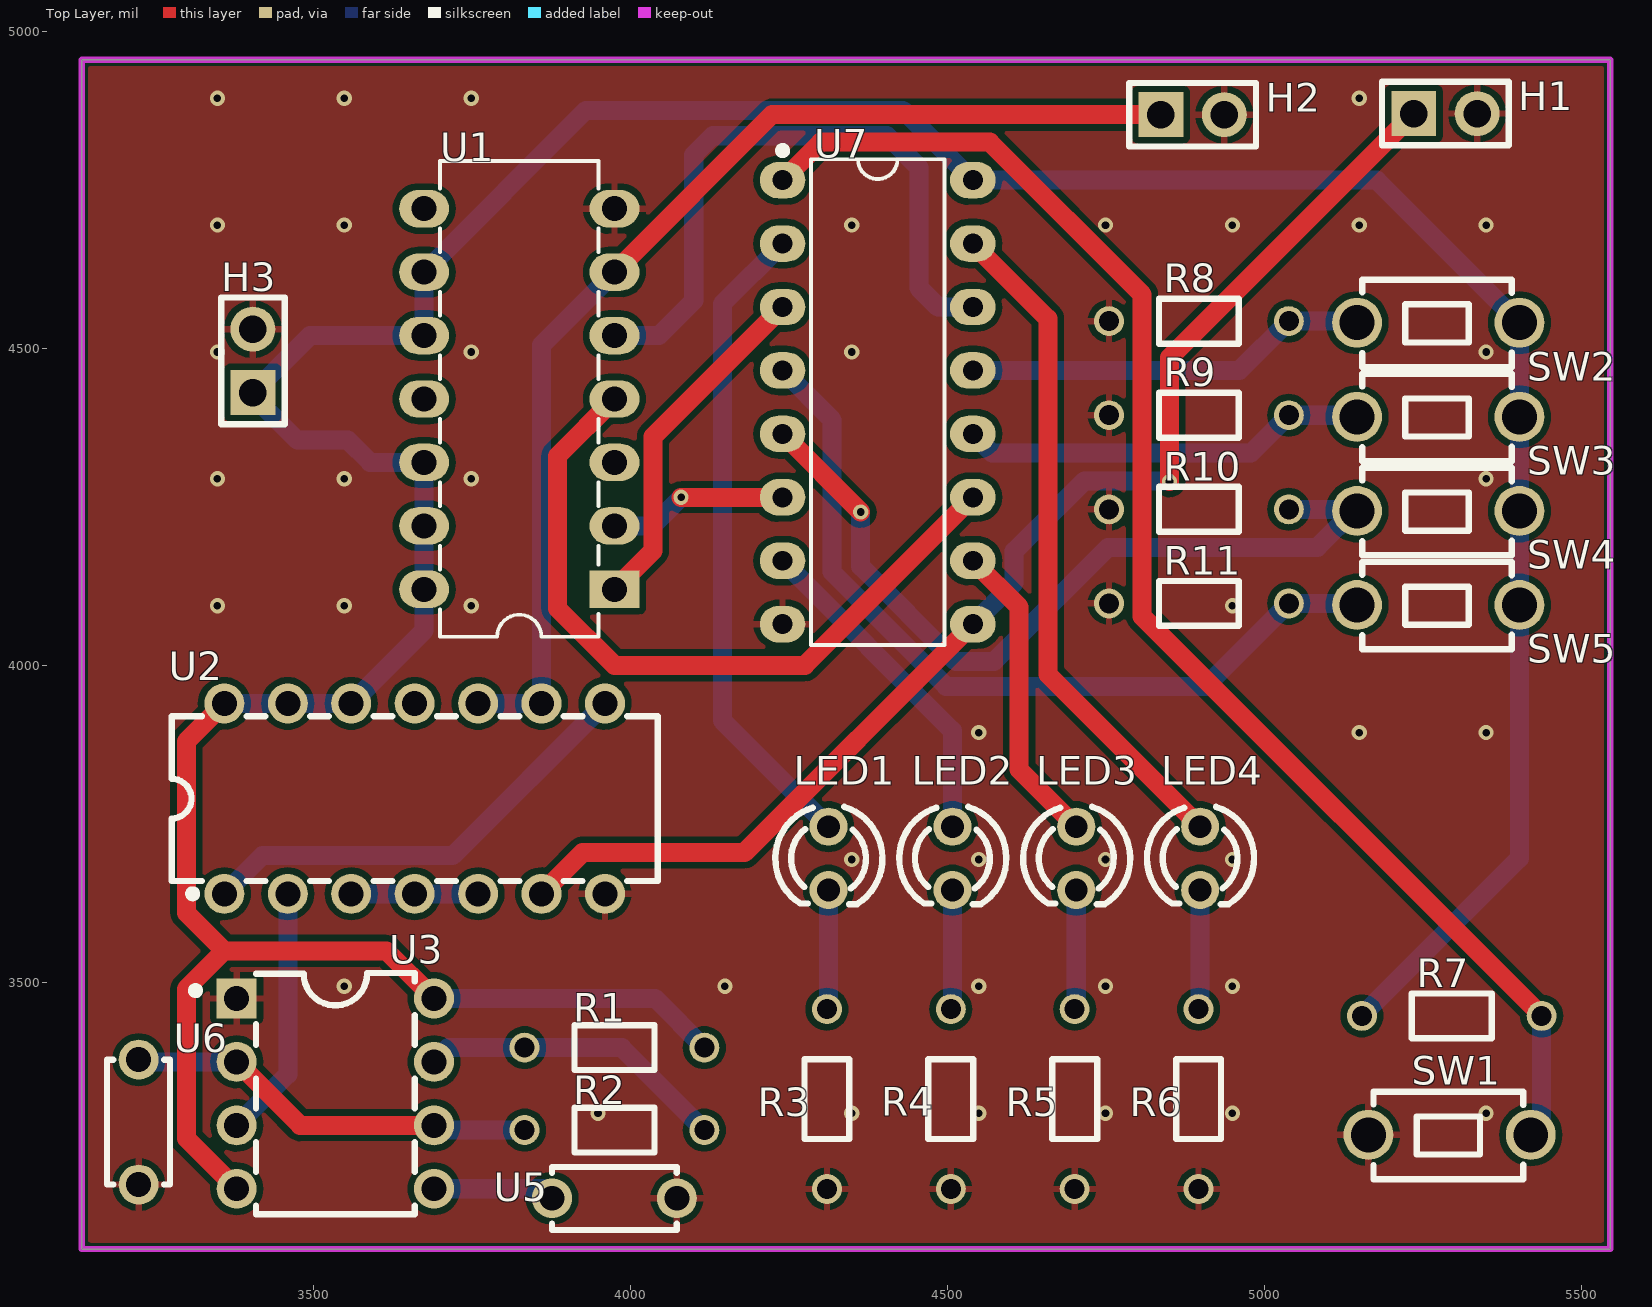
[diagram p0: Top Layer view]
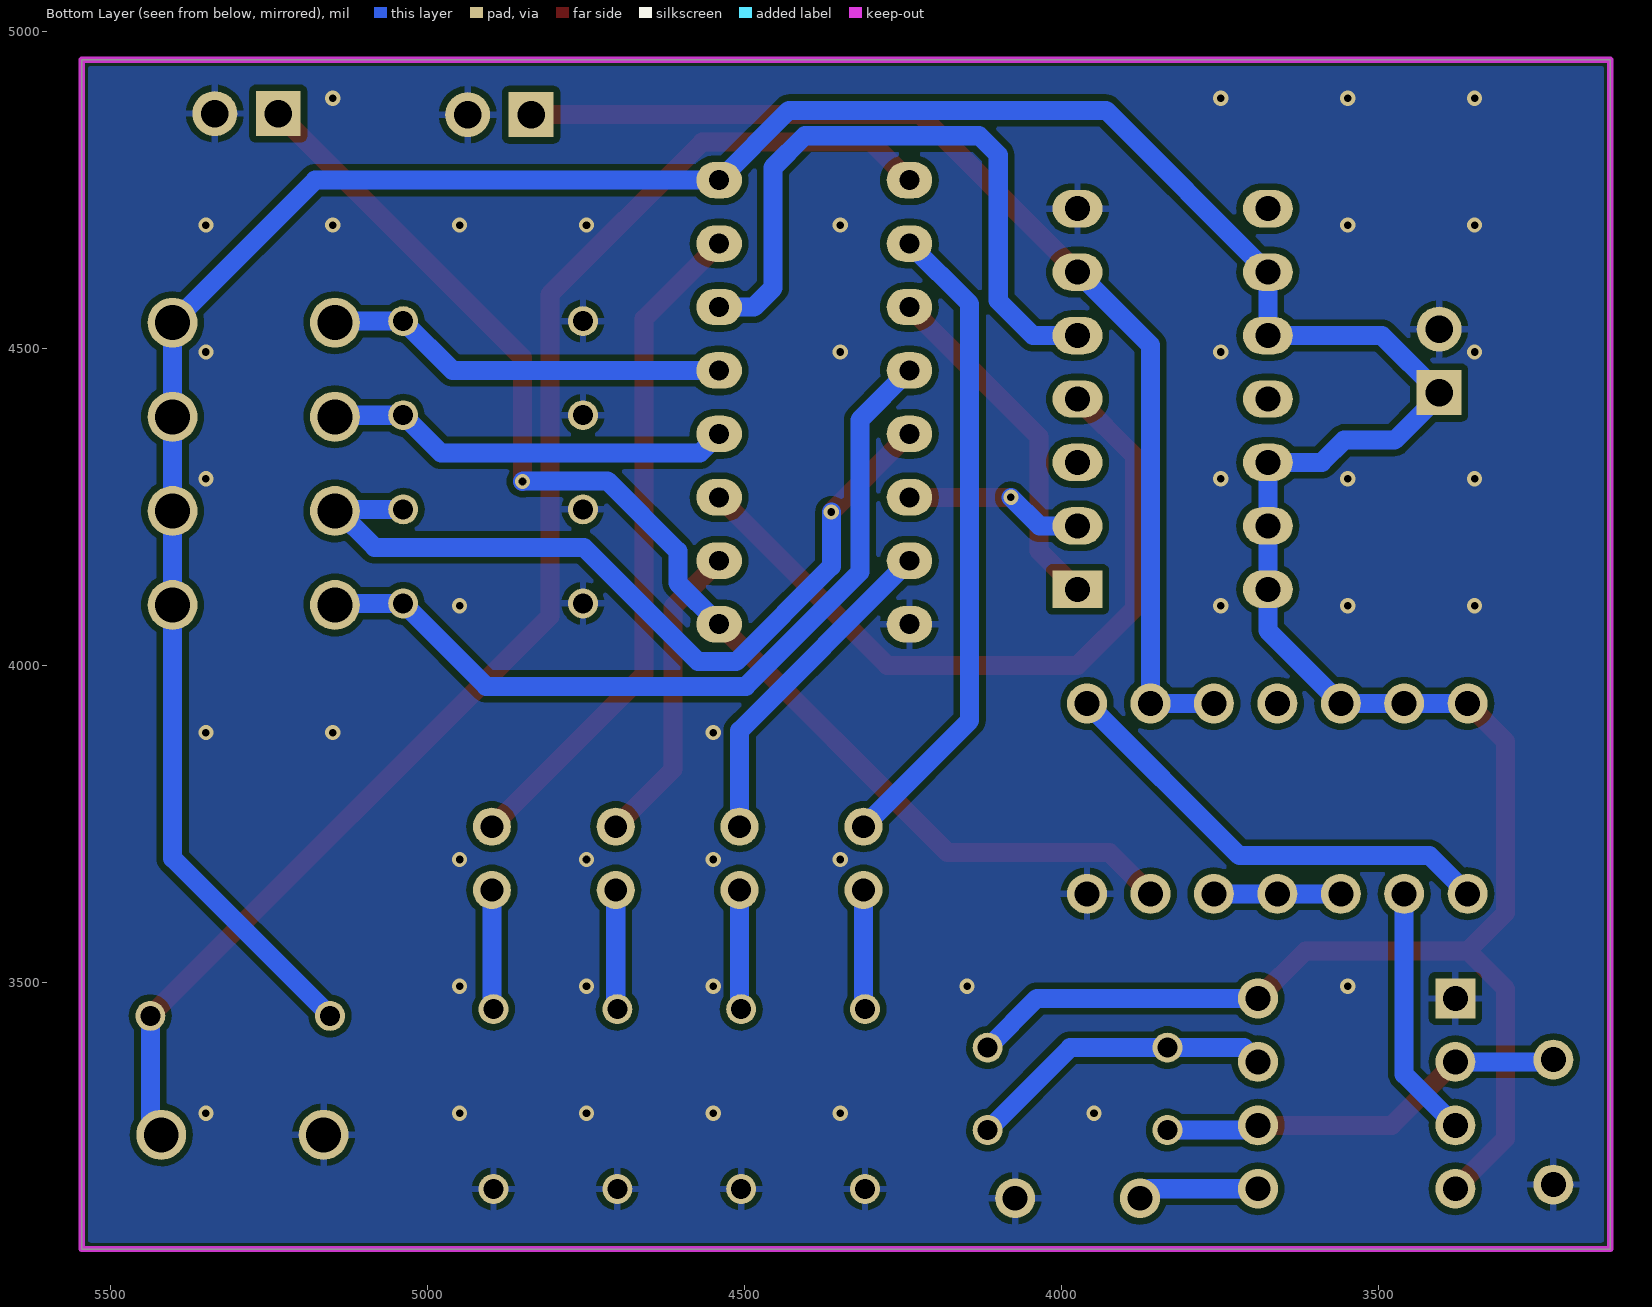
[diagram p1: Bottom Layer view, seen from below]
# Altium PCB MISC49856.pcbdoc
Units mil, origin at the board's own origin, x right, y up, seen from the top; angles counter-clockwise.
Board outline 2410 x 1875 mil, 2 copper layers (Top Layer, Bottom Layer), stack 62.206 mil thick; 29 components, 27 nets, 102 pads, 44 vias.

## Layer stack, top to bottom
Top Solder Mask Layer: solder mask 0.394, Dk 3.3
Top Layer: signal copper 1.379
Dielectric1: surface 59.449, FR4, Dk 4.5
Bottom Layer: signal copper 1.378
Bottom Solder Mask Layer: solder mask 0.394, Dk 3.3

## Board outline
3135,4955 3135,3080 5545,3080 5545,4955

## Design rules (kind name [scope] priority, off if disabled: settings)
BoardOutlineClearance copperThickness2oz_1 [All] p2 off: genericclearance=7.99 ignorepadtopadclearanceinfootprint=FALSE except(0: Arc-SplitContinuation Track-SplitContinuation SMDPad-SplitContinuation THPad-SplitContinuation Via-SplitContinuation Fill-SplitContinuation Region-SplitContinuation Poly-SplitContinuation Text-SplitContinuation Hole-SplitContinuation; 5.98: Arc-CutoutEdge SMDPad-CutoutEdge THPad-CutoutEdge Via-CutoutEdge Fill-CutoutEdge Region-CutoutEdge Text-CutoutEdge; 6.93: Hole-OutlineEdge Hole-CutoutEdge; 10: Poly-OutlineEdge Poly-CutoutEdge; 11.81: Arc-OutlineEdge Track-OutlineEdge SMDPad-OutlineEdge THPad-OutlineEdge Via-OutlineEdge Fill-OutlineEdge Region-OutlineEdge Text-OutlineEdge Track-CutoutEdge)
BoardOutlineClearance copperThickness1oz_1 [All] p4: genericclearance=4.02 ignorepadtopadclearanceinfootprint=FALSE except(0: Arc-SplitContinuation Track-SplitContinuation SMDPad-SplitContinuation THPad-SplitContinuation Via-SplitContinuation Fill-SplitContinuation Region-SplitContinuation Poly-SplitContinuation Text-SplitContinuation Hole-SplitContinuation; 6: SMDPad-CutoutEdge THPad-CutoutEdge Via-CutoutEdge Fill-CutoutEdge Region-CutoutEdge Text-CutoutEdge; 6.93: Hole-OutlineEdge Hole-CutoutEdge; 10: Poly-OutlineEdge Poly-CutoutEdge; 11.8: Arc-OutlineEdge Track-OutlineEdge SMDPad-OutlineEdge THPad-OutlineEdge Via-OutlineEdge Fill-OutlineEdge Region-OutlineEdge Text-OutlineEdge; 11.81: Arc-CutoutEdge Track-CutoutEdge)
Clearance copperThickness2oz [All] p1 off: gap=7.99 ignorepadtopadclearanceinfootprint=FALSE except(5.98: SMDPad-Track SMDPad-SMDPad THPad-Track SMDPad-THPad THPad-THPad Track-Via SMDPad-Via THPad-Via Via-Via Fill-Track Region-Track Fill-SMDPad Region-SMDPad Fill-THPad Region-THPad Fill-Via Region-Via Fill-Fill Fill-Region Region-Region Arc-Track Arc-SMDPad Arc-THPad Arc-Via Fill-Arc Region-Arc Arc-Arc Text-Track SMDPad-Text Text-THPad Text-Via Fill-Text Region-Text Arc-Text Text-Text; 6.93: Hole-Track Hole-SMDPad Hole-THPad Hole-Via Fill-Hole Region-Hole Hole-Arc Hole-Text; 10: Poly-Track Poly-SMDPad Poly-THPad Poly-Via Poly-Fill Poly-Region Poly-Poly Poly-Arc Poly-Text Poly-Hole)
Clearance copperThickness1oz [All] p3: gap=4.02 ignorepadtopadclearanceinfootprint=FALSE except(5.98: SMDPad-Track SMDPad-SMDPad THPad-Track SMDPad-THPad THPad-THPad Track-Via SMDPad-Via THPad-Via Via-Via Fill-Track Region-Track Fill-SMDPad Region-SMDPad Fill-THPad Region-THPad Fill-Via Region-Via Fill-Fill Fill-Region Region-Region; 6: Arc-Track Arc-SMDPad Arc-THPad Arc-Via Fill-Arc Region-Arc Arc-Arc Text-Track SMDPad-Text Text-THPad Text-Via Fill-Text Region-Text Arc-Text Text-Text; 6.93: Hole-Track Hole-SMDPad Hole-THPad Hole-Via Fill-Hole Region-Hole Hole-Arc Hole-Text; 10: Poly-Track Poly-SMDPad Poly-THPad Poly-Via Poly-Fill Poly-Region Poly-Poly Poly-Arc Poly-Text Poly-Hole)
Creepage creepage [All] p1: checkdistance=0 ignoreinternallayers=TRUE applytopolygonpour=TRUE
DiffPairsRouting differentialPair [All] p1: maxlimit=6 minlimit=6 mostfreqgap=6 toplayer_minwidth=5 toplayer_prefwidth=10 toplayer_maxwidth=100 toplayer_mingap=6 toplayer_prefgap=6 toplayer_maxgap=6 bottomlayer_minwidth=5 bottomlayer_prefwidth=10 bottomlayer_maxwidth=100 bottomlayer_mingap=6 bottomlayer_prefgap=6 bottomlayer_maxgap=6 maxuncoupledlength=10
HoleToHoleClearance otherClearance [All] p1: gap=11.81 allowstackedmicrovias=TRUE
Length netLength [All] p1: minlimit=0 maxlimit=0
MatchedLengths netLengthTolerance [All] p1: tolerance=1000
PasteMaskExpansion pasteMaskExpansion [All] p1: expansion=0
PlaneConnect innerPlane [All] p1: planeconnectstyle=Relief reliefexpansion=20 reliefentries=4 reliefconductorwidth=10 reliefairgap=10
PolygonConnect copperRegion [(InNet('GND'))] p1: connectstyle=Relief reliefconductorwidth=10 reliefentries=4 polygonreliefangle="90 Angle" airgapwidth=10 via.connectstyle=Relief via.reliefconductorwidth=10 via.reliefentries=4 via.polygonreliefangle="90 Angle" via.airgapwidth=10
RoutingVias viaSize [All] p1: holewidth=12.01 width=24.02 viastyle="Through Hole" minholewidth=11.81 minwidth=19.68 maxholewidth=248.03 maxwidth=393.7
SolderMaskExpansion solderMaskExpansion [IsVia] p1: expansion=-1000 istentingtop=TRUE
SolderMaskExpansion solderMaskExpansion [All] p2: expansion=2 istentingtop=FALSE
Width copperThickness2oz_2 [All] p1 off: maxlimit=100 minlimit=8 preferedwidth=10
Width copperThickness1oz_2 [All] p2: maxlimit=10 minlimit=10 preferedwidth=10 toplayer_minwidth=30 toplayer_maxwidth=100 toplayer_prefwidth=30 bottomlayer_minwidth=30 bottomlayer_maxwidth=100 bottomlayer_prefwidth=30

## Components (designator, comment, footprint, x,y, rotation, side; value= is the part's Value field where it differs from the comment)
H1 "" HDR-TH_2P-P2.54-V-M-1 5285,4870 r0 top
H2 "" HDR-TH_2P-P2.54-V-M-1 4886.33,4868.15 r0 top
H3 "" HDR-TH_2P-P2.54-V-M-1 3405,4480 r90 top
LED1 "" LED_TH-3mm 4312.42,3695.79 r270 top
LED2 "" LED_TH-3mm 4507.71,3695.79 r270 top
LED3 "" LED_TH-3mm 4702.99,3695.79 r270 top
LED4 "" LED_TH-3mm 4898.28,3695.79 r270 top
R1 "4.3kΩ" Res_1/8W 3975,3395 r0 top
R2 "5.1kΩ" Res_1/8W 3975,3265 r0 top
R3 "220Ω" Res_1/8W 4312.42,3316.4 r90 top
R4 "220Ω" Res_1/8W 4507.71,3316.4 r90 top
R5 "220Ω" Res_1/8W 4702.99,3316.4 r90 top
R6 "220Ω" Res_1/8W 4898.28,3316.4 r90 top
R7 "10kΩ" Res_1/8W 5295,3445 r0 top
R8 "10kΩ" Res_1/8W 4896.35,4540.24 r0 top
R9 "10kΩ" Res_1/8W 4896.35,4391.91 r0 top
R10 "10kΩ" Res_1/8W 4896.35,4243.59 r0 top
R11 "10kΩ" Res_1/8W 4896.35,4095.26 r0 top
SW1 "" Key_TH_3.5x6x4.3 5285,3260 r0 top
SW2 "" Key_TH_3.5x6x4.3 5267.12,4540.24 r0 top
SW3 "" Key_TH_3.5x6x4.3 5267.12,4391.91 r0 top
SW4 "" Key_TH_3.5x6x4.3 5267.12,4243.59 r0 top
SW5 "" Key_TH_3.5x6x4.3 5267.12,4095.26 r0 top
U1 "SN74LS20N(XBLW)" DIP-14_L19.0-W6.4-P2.54-LS7.6-BL 3825,4420 r90 top
U2 "SN74LS00NE4" PDIP-14_L19.3-W6.4-P2.54-LS7.9-BL 3660,3790 r0 top
U3 "LM555CM" PDIP-8_L9.6-W6.4-P2.54-LS7.9-BL-1 3535,3325 r270 top
U5 "10nF" CAP-TH_L5.0-W2.5-P5.00-D1.0 3975,3160 r0 top
U6 "100nF" CAP-TH_L5.0-W2.5-P5.00-D1.0 3225,3280 r270 top
U7 "SN74LS175N" DIP-16_L19.3-W6.4-P2.54-LS7.6-BL 4390,4415 r270 top

## Footprints (in the part's own frame and the unit in brackets; to place one, negate y for a bottom-side part, rotate by r counter-clockwise, add the part's x,y. Pads: shape width x height; smd on the part's side, far side on the other; paste and mask are expansions set on the pad)
CAP-TH_L5.0-W2.5-P5.00-D1.0 [mm]
  round 1.6 hole 1: 1(-2.5,0) 2(2.5,0)
  silkscreen extent -2.5,-1.27 2.5,1.25
DIP-14_L19.0-W6.4-P2.54-LS7.6-BL [mm]
  rect 1.5x2 hole 1: 1(-7.62,-3.81)
  oval 1.5x2 hole 1: 2(-5.08,-3.81) 3(-2.54,-3.81) 4(0,-3.81) 5(2.54,-3.81) 6(5.08,-3.81) 7(7.62,-3.81) 8(7.62,3.81) 9(5.08,3.81) 10(2.54,3.81) 11(0,3.81) 12(-2.54,3.81) 13(-5.08,3.81) 14(-7.62,3.81)
  silkscreen extent -9.53,-3.18 9.53,3.18
DIP-16_L19.3-W6.4-P2.54-LS7.6-BL [mm]
  oval 1.46x1.825 hole 0.8: 1(-8.89,-3.81) 2(-6.35,-3.81) 3(-3.81,-3.81) 4(-1.27,-3.81) 5(1.27,-3.81) 6(3.81,-3.81) 7(6.35,-3.81) 8(8.89,-3.81) 9(8.89,3.81) 10(6.35,3.81) 11(3.81,3.81) 12(1.27,3.81) 13(-1.27,3.81) 14(-3.81,3.81) 15(-6.35,3.81) 16(-8.89,3.81)
  silkscreen extent -10.22,-3.96 9.73,2.67
HDR-TH_2P-P2.54-V-M-1 [mm]
  rect 1.8x1.8 hole 1.1: 1(-1.27,0)
  round 1.8 hole 1.1: 2(1.27,0)
  silkscreen extent -2.54,-1.27 2.54,1.27
Key_TH_3.5x6x4.3 [mil]
  round 78.7 hole 55.1 paste+0 mask+2: A(-121.44,0) B(134.46,0)
  silkscreen extent -114,-70 123,68
LED_TH-3mm [mil]
  round 60 hole 36 paste+0 mask+2: 1(-50,0) 2(50,0)
  silkscreen extent -81,-84 72,85
PDIP-8_L9.6-W6.4-P2.54-LS7.9-BL-1 [mil]
  rect 63x63 hole 39.37: 1(-150,-155.51)
  round 63 hole 39.37: 2(-50,-155.51) 3(50,-155.51) 4(150,-155.51) 5(150,155.52) 6(50,155.52) 7(-50,155.52) 8(-150,155.52)
  silkscreen extent -190,-226 190,125
PDIP-14_L19.3-W6.4-P2.54-LS7.9-BL [mm]
  round 1.6 hole 1: 1(-7.62,-3.81) 2(-5.08,-3.81) 3(-2.54,-3.81) 4(0,-3.81) 5(2.54,-3.81) 6(5.08,-3.81) 7(7.62,-3.81) 8(7.62,3.81) 9(5.08,3.81) 10(2.54,3.81) 11(0,3.81) 12(-2.54,3.81) 13(-5.08,3.81) 14(-7.62,3.81)
  silkscreen extent -9.73,-3.96 9.73,3.3
Res_1/8W [mil]
  round 47.2 hole 31.5 paste+0 mask+2: 1(-141.7,2.48) 2(141.7,2.48)
  silkscreen extent -63,-33 63,38

## Via types
v1: diameter 24.02, hole 12, Top Layer to Bottom Layer, 44 vias

## Nets (pads, with @x,y where several pads share a name; then routed paths per layer and width w, separated by ;. In a path a pad name is that pad's centre, name@x,y a point inside that pad or via, vN(x,y) a via of type N, cw(c..) or ccw(c..) an arc to the next point about the centre after c; other vN are vias at no path point)
$1N1: U2.2 U3.3 | length 398.3
  Bottom Layer w30: U3.3 3460,3355.52 U2.2
$1N2: R1.1 R2.2 U3.7 | length 489.3
  Bottom Layer w30: U3.7 3712.99,3397.48 R1.1 3986.7,3397.48 R2.2
$1N4: R2.1 U3.2 U3.6 U6.1 | length 654.3
  Top Layer w30: U3.2 3479.49,3275 U3.6
  Bottom Layer w30: U6.1 3228.42,3375 U3.2 ; U3.6 3698.03,3267.48 R2.1
$1N5: U3.5 U5.1 | length 192.3
  Bottom Layer w30: U3.5 3861.58,3175 U5.1
$1N7: LED1.2 R3.2 | length 188.7
  Bottom Layer w30: R3.2 4312.42,3460.58 LED1.2
$1N8: LED2.2 R4.2 | length 188.7
  Bottom Layer w30: R4.2 4507.71,3460.58 LED2.2
$1N9: LED3.2 R5.2 | length 188.7
  Bottom Layer w30: R5.2 4702.99,3460.58 LED3.2
$1N10: LED4.2 R6.2 | length 188.7
  Bottom Layer w30: R6.2 4898.28,3460.58 LED4.2
$1N11: LED4.1 U7.15 | length 1067.6
  Top Layer w30: U7.15 4658.28,4546.72 4658.28,3985.79 LED4.1
$1N12: LED3.1 U7.10 | length 486.7
  Top Layer w30: U7.10 4612.99,4092.01 4612.99,3835.79 LED3.1
$1N13: LED2.1 U7.7 | length 530.1
  Bottom Layer w30: U7.7 4507.71,3897.29 LED2.1
$1N14: LED1.1 U7.2 | length 1027.9
  Bottom Layer w30: U7.2 4145,4570 4145,3913.21 LED1.1
$1N15: U1.1 U7.3 | length 554.8
  Top Layer w30: U1.1 4035.75,4180.75 4035.75,4360.75 U7.3
$1N16: U1.2 U7.6 | length 283.6
  Top Layer w30: v1(4080,4265) U7.6
  Bottom Layer w30: U1.2 4035,4220 v1(4080,4265)
$1N17: U1.4 U7.11 | length 1169.3
  Top Layer w30: U1.4 3885,4330 3885,4090 3975,4000 4275,4000 U7.11
$1N18: U1.5 U7.14 | length 1053.3
  Bottom Layer w30: U1.5 4045,4520 4100,4575 4100,4805 4130,4835 4210.77,4835 4405,4835 4455,4785 4455,4595 4485,4565 U7.14
$1N19: R7.2 SW1.B U7.1 | length 2284.1
  Top Layer w30: U7.1 4300,4825 4566.7,4825 4806.7,4585 4806.7,4077.47 R7.2
  Bottom Layer w30: SW1.B 5436.7,3277.24 R7.2
$1N20: H1.1 U2.6 U7.9 | length 2028.5
  Top Layer w30: U2.6 3925.01,3705 4180,3705 U7.9 ; v1(4850,4290) 4850,4485 H1.1
  Bottom Layer w30: U7.9 4605,4130 4605,4180 4715.65,4290.65 4849.35,4290.65 v1(4850,4290)
$1N22: H2.1 U1.6 U2.9 U2.10 | length 1791.8
  Top Layer w30: U1.6 4223.15,4868.15 H2.1@4836.33,4868.15
  Bottom Layer w30: U2.10 U2.9 3860,4505 U1.6
$1N23: U2.1 U2.8 | length 724.3
  Bottom Layer w30: U2.1 3420,3700 3720,3700 U2.8
$1N26: U2.3 U2.4 U2.5 | length 200
  Bottom Layer w30: U2.3 U2.4 U2.5
$1N28: R9.2 SW3.A U7.12 | length 643.7
  Bottom Layer w30: U7.12 4570,4335 4978.66,4335 5038.05,4394.39 5143.2,4394.39 SW3.A
$1N30: R8.2 SW2.A U7.13 | length 638.9
  Bottom Layer w30: U7.13 4960.34,4465 5038.05,4542.71 5143.2,4542.71 SW2.A
$1N31: R10.2 SW4.A U7.5 | length 1310.2
  Top Layer w30: U7.5 v1(4363.21,4241.8)
  Bottom Layer w30: v1(4363.21,4241.8) 4363.21,4156.06 4513.2,4006.06 4573.2,4006.06 4753.2,4186.06 5083.2,4186.06 SW4.A@5143.2,4246.06 ; R10.2@5038.05,4246.06 SW4.A@5143.2,4246.06 ; SW4.A SW4.A@5143.2,4246.06
$1N32: R11.2 SW5.A U7.4 | length 1307.8
  Bottom Layer w30: U7.4 4318.05,4386.95 4318.05,4146.95 4498.05,3966.95 4907.27,3966.95 5038.05,4097.73 5143.2,4097.73 SW5.A
GND: H1.2 H2.2 H3.2 R3.1 R4.1 R5.1 R6.1 R8.1 R9.1 R10.1 R11.1 SW1.A U1.7 U2.7 U3.1 U5.2 U6.2 U7.8
  other v1: 3949.1,3294.1 4349.1,3294.1 4549.1,3294.1 4749.1,3294.1 4949.1,3294.1 5349.1,3294.1 3549.1,3494.1 4149.1,3494.1 4549.1,3494.1 4749.1,3494.1 4949.1,3494.1 4349.1,3694.1 4549.1,3694.1 4749.1,3694.1 4949.1,3694.1 4549.1,3894.1 5149.1,3894.1 5349.1,3894.1 3349.1,4094.1 3549.1,4094.1 3749.1,4094.1 4949.1,4094.1 3349.1,4294.1 3549.1,4294.1 3749.1,4294.1 5349.1,4294.1 3349.1,4494.1 3749.1,4494.1 4349.1,4494.1 5349.1,4494.1 3349.1,4694.1 3549.1,4694.1 4349.1,4694.1 4749.1,4694.1 4949.1,4694.1 5149.1,4694.1 5349.1,4694.1 3349.1,4894.1 3549.1,4894.1 3749.1,4894.1 5149.1,4894.1
VCC: H3.1 R1.2 R7.1 SW2.B SW3.B SW4.B SW5.B U1.9 U1.10 U1.12 U1.13 U1.14 U2.12 U2.13 U2.14 U3.4 U3.8 U7.16 | length 6212.2
  Top Layer w30: U2.14 3300,3880 3300,3610 3360,3550 ; U3.4 3300,3254.48 3300,3490 3360,3550 ; U3.8 3615.51,3550 3360,3550
  Bottom Layer w30: U2.14 U2.13 U2.12 3675,4055 U1.14 U1.13 U1.12 3590,4320 3555,4355 3475,4355 3405,4425 H3.1 3495,4520 U1.10 U1.9 3930,4875 4430,4875 U7.16 5176.82,4765 SW2.B SW3.B SW4.B SW5.B 5401.58,3695.76 R7.1 ; U3.8 4039.18,3475 R1.2
pads on no net: U1.3 U1.8 U1.11 U2.11

## Polygon pours and split planes (outlines as drawn)
GND on Top Layer (solid, remove dead copper, pour order 0): 3050,4995 3050,3020 5680,3020 5680,4995
GND on Bottom Layer (solid, remove dead copper, pour order 2): 3000,5030 3000,3000 5735,3000 5735,5030

## Keep-outs
Board Outline Layer:
  the board outline again, w10

## Silkscreen, mask and mechanical layers (free items; w line width, h text height)
Top Silkscreen Layer: